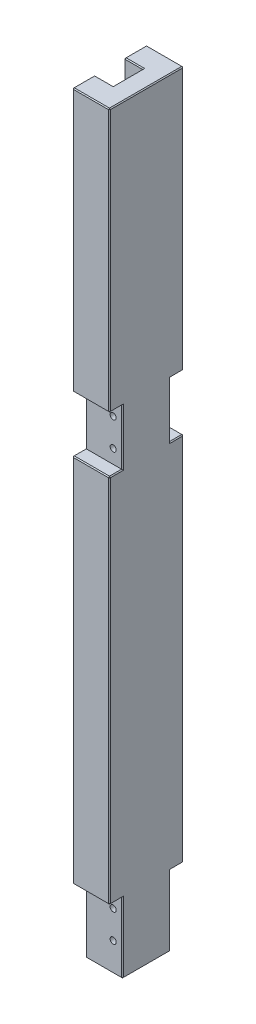
from build123d import *

# Parameters (mm, degrees)
SKETCH_1_W          = 40
SKETCH_1_H          = 410
EXTRUDE_1_DEPTH     = 20
SKETCH_2_W          = 16
SKETCH_2_H          = 410
CUT_EXTRUDE_1_DEPTH = 10
SKETCH_3_W          = 20
SKETCH_3_H          = 38
SKETCH_3_H_2        = 30
CUT_EXTRUDE_2_DEPTH = 7
SKETCH_4_W          = 20
SKETCH_4_H          = 30
SKETCH_4_H_2        = 38
CUT_EXTRUDE_3_DEPTH = 7
HOLE_WIZARD_M4_1_D  = 3.3
CHAMFER_1_SIZE      = 0.5


with BuildPart() as part:
    # 草图1 → 凸台-拉伸1 (new body)
    with BuildSketch(Plane(origin=(0, 0, 0), x_dir=(0, 0, -1), z_dir=(1, 0, 0))):
        Rectangle(SKETCH_1_W, SKETCH_1_H)
    extrude(amount=EXTRUDE_1_DEPTH)

    # 草图2 → 切除-拉伸1 (cut)
    with BuildSketch(Plane.ZY):
        Rectangle(SKETCH_2_W, SKETCH_2_H)
    extrude(amount=-CUT_EXTRUDE_1_DEPTH, mode=Mode.SUBTRACT)

    # 草图3 → 切除-拉伸2 (cut)
    with BuildSketch(Plane.XY.offset(20)):
        with Locations((10, -186)):
            Rectangle(SKETCH_3_W, SKETCH_3_H)
        with Locations((10, 48)):
            Rectangle(SKETCH_3_W, SKETCH_3_H_2)
    extrude(amount=-CUT_EXTRUDE_2_DEPTH, mode=Mode.SUBTRACT)

    # 草图4 → 切除-拉伸3 (cut)
    with BuildSketch(Plane(origin=(0, 0, -20), x_dir=(-1, 0, 0), z_dir=(0, 0, -1))):
        with Locations((-10, 48)):
            Rectangle(SKETCH_4_W, SKETCH_4_H)
        with Locations((-10, -186)):
            Rectangle(SKETCH_4_W, SKETCH_4_H_2)
    extrude(amount=-CUT_EXTRUDE_3_DEPTH, mode=Mode.SUBTRACT)

    # M4 螺纹孔1 (through all)
    with Locations(Plane(origin=(0, 0, -13), x_dir=(-1, 0, 0), z_dir=(0, 0, -1))):
        with Locations((-15, 55.5), (-15, 40.5), (-15, -174.49792687), (-15, -189.49792687)):
            Hole(HOLE_WIZARD_M4_1_D / 2)

    # 倒角1
    chamfer_1_edges = [part.edges().sort_by_distance(p)[0] for p in [
        (20, 134, 20),
        (0, -205, -10.5),
        (0, 205, 14),
        (5, 205, 8),
        (10, -205, 0),
        (5, -205, 8),
        (5, -205, -8),
        (10, 205, 0),
        (5, 205, -8),
        (0, 0, 8),
        (0, 0, -8),
        (20, -205, 0),
        (0, -205, 10.5),
        (0, -186, 13),
        (0, -167, 16.5),
        (20, -186, 13),
        (20, -167, 16.5),
        (10, -205, 13),
        (10, -167, 20),
        (20, -67, 20),
        (0, -67, 20),
        (0, 48, 13),
        (0, 33, 16.5),
        (0, 63, 16.5),
        (20, 48, 13),
        (20, 63, 16.5),
        (20, 33, 16.5),
        (0, 134, 20),
        (10, 33, 20),
        (10, 63, 20),
        (0, 205, -14),
        (0, 134, -20),
        (20, 134, -20),
        (0, 48, -13),
        (0, 63, -16.5),
        (0, 33, -16.5),
        (20, 48, -13),
        (20, 33, -16.5),
        (20, 63, -16.5),
        (10, 63, -20),
        (10, 33, -20),
        (20, 205, 0),
        (0, -67, -20),
        (20, -67, -20),
        (10, 205, 20),
        (0, -186, -13),
        (0, -167, -16.5),
        (10, 205, -20),
        (10, -205, -13),
        (20, -186, -13),
        (20, -167, -16.5),
        (10, -167, -20),
    ]]
    chamfer(chamfer_1_edges, length=CHAMFER_1_SIZE)


solid = part.part
